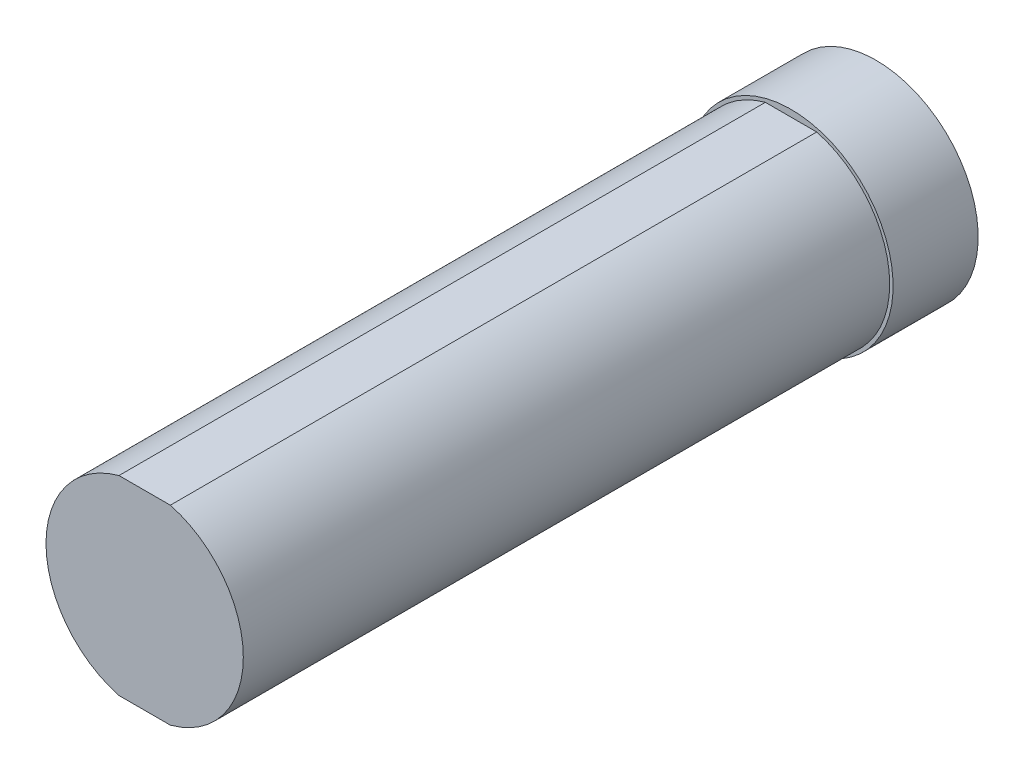
from build123d import *

# Parameters (mm, degrees)
SKETCH1_R           = 29
BOSS_EXTRUDE1_DEPTH = 190
SKETCH2_R           = 30
BOSS_EXTRUDE2_DEPTH = 25
SKETCH4_OUTSIDE_W   = 108.228
SKETCH4_OUTSIDE_H   = 108.228
SKETCH4_OUTSIDE_W_2 = 84.198703348
SKETCH4_OUTSIDE_H_2 = 56
CUT_EXTRUDE1_DEPTH  = 190
SKETCH5_R           = 24
CUT_EXTRUDE2_DEPTH  = 22
SKETCH6_R           = 24.1
CUT_EXTRUDE3_DEPTH  = 3
SKETCH7_R           = 18
CUT_EXTRUDE4_DEPTH  = 180
SKETCH8_R           = 5
SKETCH8_R_2         = 7.5
CUT_EXTRUDE5_DEPTH  = 180
CHAMFER1_SIZE       = 1


with BuildPart() as part:
    # Sketch1 → Boss-Extrude1 (new body)
    with BuildSketch(Plane.XY):
        Circle(SKETCH1_R)
    extrude(amount=BOSS_EXTRUDE1_DEPTH)

    # Sketch2 → Boss-Extrude2 (add)
    with BuildSketch(Plane(origin=(0, 0, 0), x_dir=(-1, 0, 0), z_dir=(0, 0, -1))):
        Circle(SKETCH2_R)
    extrude(amount=BOSS_EXTRUDE2_DEPTH)

    # Sketch4 outside → Cut-Extrude1 (cut)
    with BuildSketch(Plane.XY.offset(190)):
        Rectangle(SKETCH4_OUTSIDE_W, SKETCH4_OUTSIDE_H)
        Rectangle(SKETCH4_OUTSIDE_W_2, SKETCH4_OUTSIDE_H_2, mode=Mode.SUBTRACT)
    extrude(amount=-CUT_EXTRUDE1_DEPTH, mode=Mode.SUBTRACT)

    # Sketch5 → Cut-Extrude2 (cut)
    with BuildSketch(Plane(origin=(0, 0, -25), x_dir=(-1, 0, 0), z_dir=(0, 0, -1))):
        Circle(SKETCH5_R)
    extrude(amount=-CUT_EXTRUDE2_DEPTH, mode=Mode.SUBTRACT)

    # Sketch6 → Cut-Extrude3 (cut)
    with BuildSketch(Plane(origin=(0, 0, -3), x_dir=(-1, 0, 0), z_dir=(0, 0, -1))):
        Circle(SKETCH6_R)
    extrude(amount=-CUT_EXTRUDE3_DEPTH, mode=Mode.SUBTRACT)

    # Sketch7 → Cut-Extrude4 (cut)
    with BuildSketch(Plane(origin=(0, 0, 0), x_dir=(-1, 0, 0), z_dir=(0, 0, -1))):
        Circle(SKETCH7_R)
    extrude(amount=-CUT_EXTRUDE4_DEPTH, mode=Mode.SUBTRACT)

    # Sketch8 → Cut-Extrude5 (cut)
    with BuildSketch(Plane(origin=(0, 0, 0), x_dir=(1, 0, 0), z_dir=(0, 1, 0))):
        with Locations(Location((0, -55, 0), (0, 0, 270))):
            Circle(SKETCH8_R)
        with Locations(Location((0, -130, 0), (0, 0, 270))):
            Circle(SKETCH8_R_2)
    extrude(amount=-CUT_EXTRUDE5_DEPTH, mode=Mode.SUBTRACT)

    # Chamfer1
    chamfer1_edges = [part.edges().sort_by_distance(p)[0] for p in [
        (24, 0, -25),
    ]]
    chamfer(chamfer1_edges, length=CHAMFER1_SIZE)


solid = part.part
